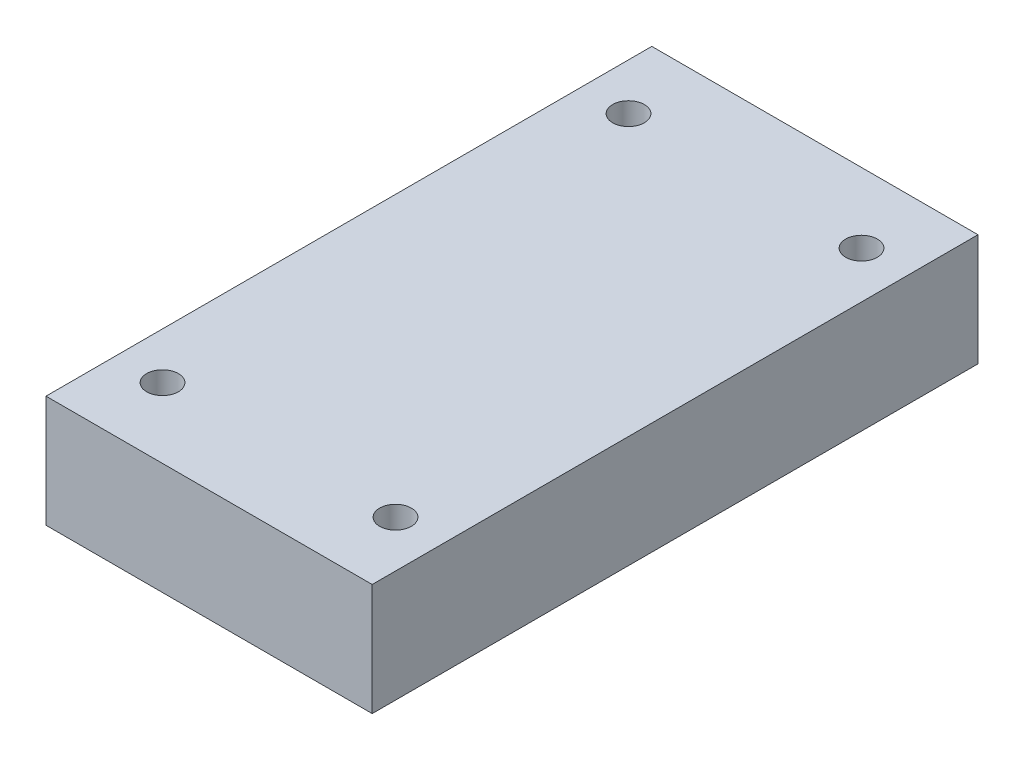
from build123d import *

# Parameters (mm, degrees)
SKETCH_1_W         = 70
SKETCH_1_H         = 130
EXTRUDE_1_DEPTH    = 24
HOLE_WIZARD_M8_1_D = 6.8


with BuildPart() as part:
    # 草图1 → 凸台-拉伸1 (new body)
    with BuildSketch(Plane(origin=(0, 0, 0), x_dir=(1, 0, 0), z_dir=(0, 1, 0))):
        Rectangle(SKETCH_1_W, SKETCH_1_H)
    extrude(amount=EXTRUDE_1_DEPTH)

    # M8 螺纹孔1 (through all)
    with Locations(Plane(origin=(0, 24, 0), x_dir=(1, 0, 0), z_dir=(0, 1, 0))):
        with Locations((-25, -50), (-25, 50), (25, 50), (25, -50)):
            Hole(HOLE_WIZARD_M8_1_D / 2)


solid = part.part
